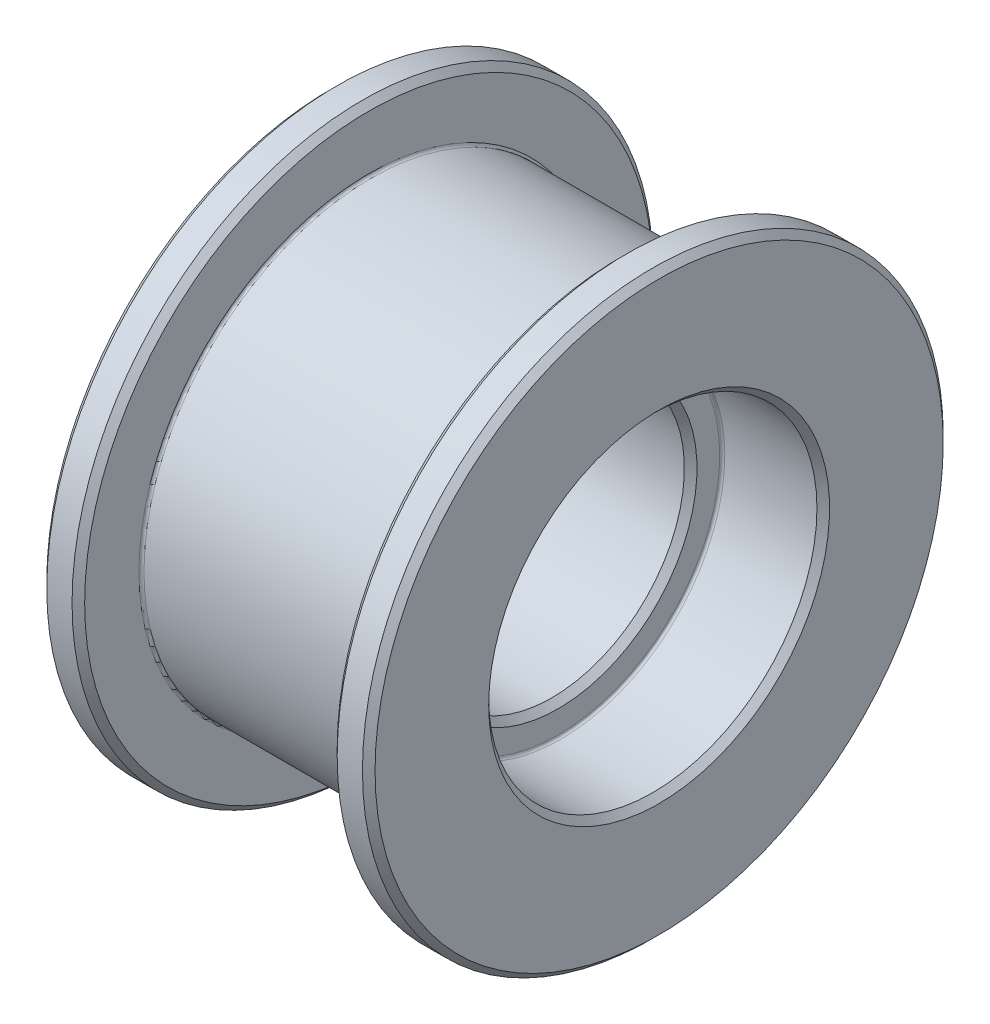
SolidWorks part; units mm, degrees
material "6061 合金"
ref_plane "前视基准面" through (0, 0, 0) normal (0, 0, 1) x (1, 0, 0)
ref_plane "上视基准面" through (0, 0, 0) normal (0, 1, 0) x (1, 0, 0)
ref_plane "右视基准面" through (0, 0, 0) normal (1, 0, 0) x (0, 0, -1)
sketch "草图1" plane through (0, 0, 0) normal (0, 0, 1) x (1, 0, 0)
  line L0 (0, 82.6549) -> (0, 0) construction
  line L1 (0, 0) -> (101.7989, 0) construction
  line L2 (-13, 13) -> (-13, 23)
  line L3 (13, 13) -> (13, 23)
  line L4 (-13, 23) -> (-10, 23)
  line L5 (13, 23) -> (10, 23)
  line L6 (-10, 23) -> (-10, 18)
  line L7 (10, 23) -> (10, 18)
  line L8 (-10, 18) -> (10, 18)
  line L9 (-13, 13) -> (-5, 13)
  line L10 (13, 13) -> (5, 13)
  line L11 (-5, 13) -> (-5, 10.5)
  line L12 (5, 13) -> (5, 10.5)
  line L13 (-5, 10.5) -> (5, 10.5)
  point P13 (0, 18)
  point P17 (0, 10.5)
  dimension "D1" = 26
  dimension "D2" = 8
  dimension "D3" = 3
  dimension "D4" = 5
  dimension "D5" = 20
  dimension "D6" = 21
  dimension "D7" = 5
revolve "旋转1" add sketch "草图1" angle 360 about L1
chamfer "倒角1" distance 0.5 angle 45 8 edges at (5, 0, 10.5) (13, 0, 13) (13, 0, 23) (10, 0, 23) (-10, 0, 23) (-5, 0, 10.5) (-13, 0, 13) (-13, 0, 23)
fillet "圆角1" radius 0.2 4 edges at (5, 0, 13) (-10, 0, 18) (10, 0, 18) (-5, 0, 13)
